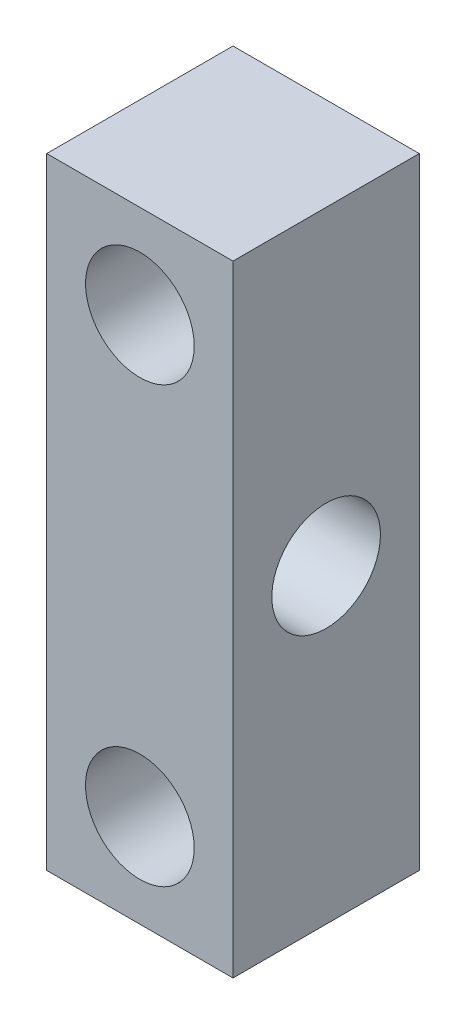
from build123d import *

# Parameters (mm, degrees)
SKETCH_1_W          = 12
SKETCH_1_H          = 40
SKETCH_1_R          = 3.5
EXTRUDE_1_DEPTH     = 6
CUT_EXTRUDE_1_REACH = 26.083
SKETCH_2_R          = 3.5


with BuildPart() as part:
    # 草图1 → 凸台-拉伸1 (new, symmetric)
    with BuildSketch(Plane.XY):
        Rectangle(SKETCH_1_W, SKETCH_1_H)
        with Locations((0, 14)):
            Circle(SKETCH_1_R, mode=Mode.SUBTRACT)
        with Locations((0, -14)):
            Circle(SKETCH_1_R, mode=Mode.SUBTRACT)
    extrude(amount=EXTRUDE_1_DEPTH, both=True)

    # 草图2 → 切除-拉伸1 (cut, up to next)
    with BuildSketch(Plane(origin=(6, 0, 0), x_dir=(0, 0, -1), z_dir=(1, 0, 0)), mode=Mode.PRIVATE) as cut_extrude_1_sk1:
        Circle(SKETCH_2_R)
    cut_extrude_1_tool1 = extrude(cut_extrude_1_sk1.sketch, amount=-CUT_EXTRUDE_1_REACH, mode=Mode.PRIVATE) & part.part
    add(cut_extrude_1_tool1.solids().sort_by_distance((6, 0, 0))[0], mode=Mode.SUBTRACT)


solid = part.part
